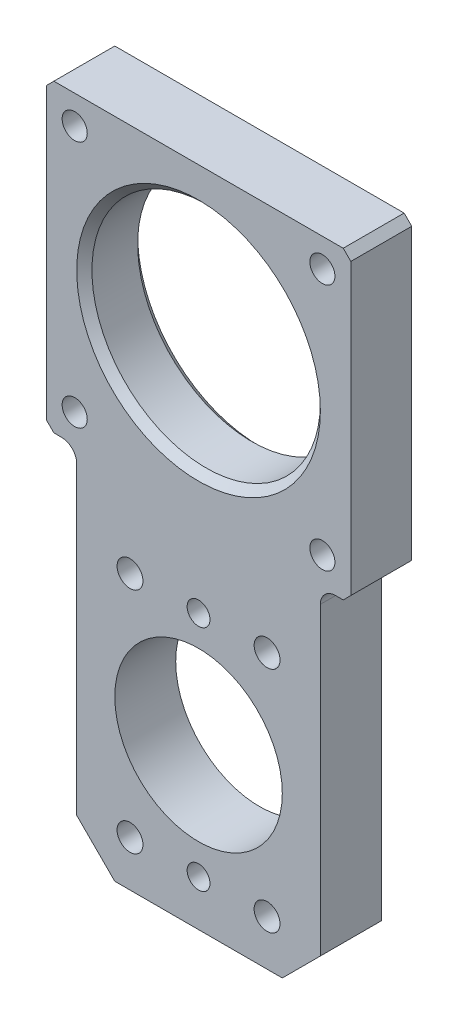
from build123d import *

# Parameters (mm, degrees)
BOSS_EXTRUDE1_DEPTH  = 4
M4_TAPPED_HOLE1_D    = 3.3
M3_CLEARANCE_HOLE1_D = 3.4
SKETCH6_R            = 15
SKETCH6_R_2          = 1.5
SKETCH6_R_3          = 11
CUT_EXTRUDE1_DEPTH   = 49.541219597
CHAMFER1_SIZE        = 5
CHAMFER2_SIZE        = 1
FILLET1_R            = 2


with BuildPart() as part:
    # Sketch1 → Boss-Extrude1 (new, symmetric)
    with BuildSketch(Plane.XY):
        Polygon((-16, 3.5), (-16, -43.5), (16, -43.5), (16, 3.5), (20, 3.5), (20, 43.5), (-20, 43.5), (-20, 3.5), align=None)
    extrude(amount=BOSS_EXTRUDE1_DEPTH, both=True)

    # M4 Tapped Hole1 (through all)
    with Locations(Plane.XY.offset(4)):
        with Locations((-16.263455967, 39.763455967), (16.263455967, 39.763455967), (16.263455967, 7.236544033), (-16.263455967, 7.236544033)):
            Hole(M4_TAPPED_HOLE1_D / 2)

    # M3 Clearance Hole1 (through all)
    with Locations(Plane.XY.offset(4)):
        with Locations((-9, -7.5), (9, -7.5), (9, -37.5), (-9, -37.5)):
            Hole(M3_CLEARANCE_HOLE1_D / 2)

    # Sketch6 → Cut-Extrude1 (cut, through all)
    with BuildSketch(Plane.XY.offset(4)):
        with Locations((0, 23.5)):
            Circle(SKETCH6_R)
        with Locations((0, -7.5)):
            Circle(SKETCH6_R_2)
        with Locations((0, -37.5)):
            Circle(SKETCH6_R_2)
        with Locations((0, -22.5)):
            Circle(SKETCH6_R_3)
    extrude(amount=-CUT_EXTRUDE1_DEPTH, mode=Mode.SUBTRACT)

    # Chamfer1
    chamfer1_edges = [part.edges().sort_by_distance(p)[0] for p in [
        (16, -43.5, 0),
        (-16, -43.5, 0),
    ]]
    chamfer(chamfer1_edges, length=CHAMFER1_SIZE)

    # Chamfer2
    chamfer2_edges = [part.edges().sort_by_distance(p)[0] for p in [
        (-20, 3.5, 0),
        (-20, 43.5, 0),
        (20, 43.5, 0),
        (20, 3.5, 0),
        (-15, 23.5, -4),
        (-15, 23.5, 4),
    ]]
    chamfer(chamfer2_edges, length=CHAMFER2_SIZE)

    # Fillet1
    fillet1_edges = [part.edges().sort_by_distance(p)[0] for p in [
        (-16, 3.5, 0),
        (16, 3.5, 0),
    ]]
    fillet(fillet1_edges, radius=FILLET1_R)


solid = part.part
